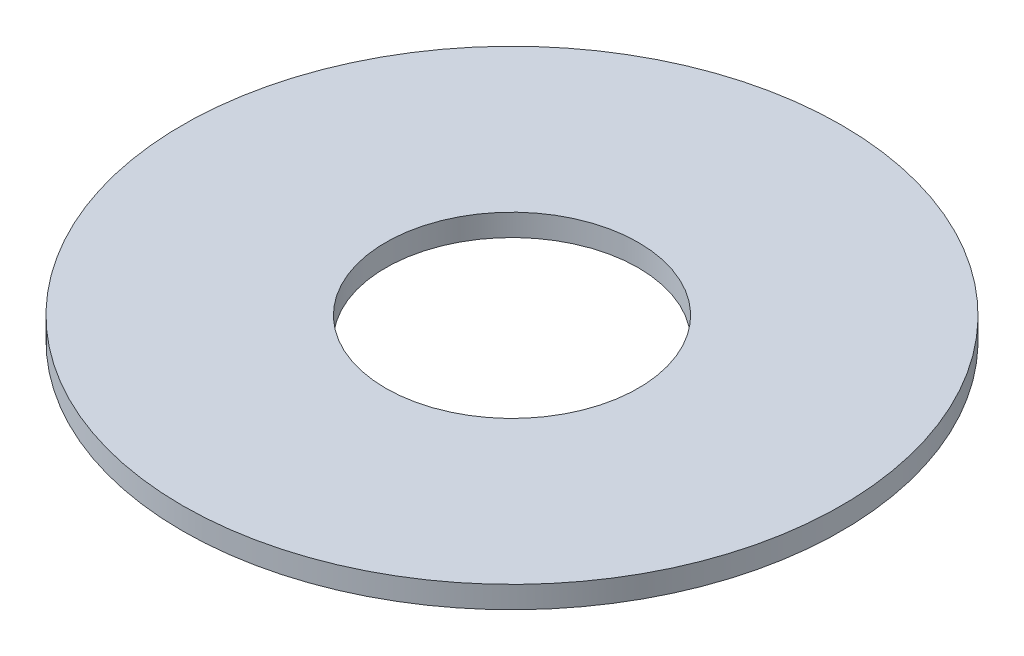
SolidWorks part; units mm, degrees
ref_plane "Front Plane" through (0, 0, 0) normal (0, 0, 1) x (1, 0, 0)
ref_plane "Top Plane" through (0, 0, 0) normal (0, 1, 0) x (1, 0, 0)
ref_plane "Right Plane" through (0, 0, 0) normal (1, 0, 0) x (0, 0, -1)
sketch "Sketch1" plane through (0, 0, 0) normal (0, 1, 0) x (1, 0, 0)
  circle A0 centre (0, 0) radius 11.5
  circle A1 centre (0, 0) radius 30
  dimension "D1" = 23
  dimension "D2" = 60
extrude "Boss-Extrude1" add sketch "Sketch1" along normal blind 2
